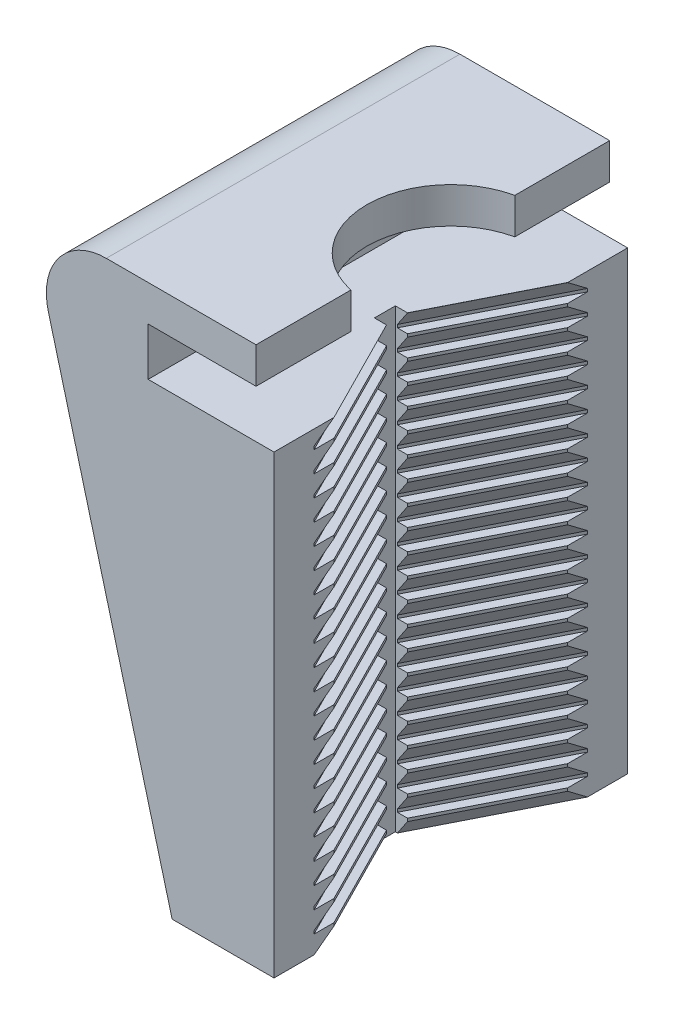
from build123d import *

# Parameters (mm, degrees)
BOSS_EXTRUDE1_DEPTH     = 59
CUT_EXTRUDE2_REACH      = 116.122
SKETCH3_R               = 14
CUT_EXTRUDE3_DEPTH      = 115.121756946
CUT_EXTRUDE3_DEPTH_BACK = 80
CUT_EXTRUDE5_DEPTH      = 80
CUT_EXTRUDE6_DEPTH      = 99.782303331
SKETCH9_W               = 3.123815153
SKETCH9_H               = 3.5
CUT_EXTRUDE7_DEPTH      = 80


with BuildPart() as part:
    # Sketch1 → Boss-Extrude1 (new body)
    with BuildSketch(Plane.XY):
        with BuildLine():
            Line((0, 0), (0, 76))
            Line((0, 76), (-21, 76))
            Line((-21, 76), (-21, 84))
            Line((-21, 84), (-3, 84))
            Line((-3, 84), (-3, 90))
            Line((-3, 90), (-27.983883536, 90))
            ThreePointArc((-27.983883536, 90), (-35.913772093, 86.092361404), (-37.646232932, 77.423373494))
            Line((-37.646232932, 77.423373494), (-17, 0))
            Line((-17, 0), (0, 0))
        make_face()
    extrude(amount=BOSS_EXTRUDE1_DEPTH)

    # Sketch3 → Cut-Extrude2 (cut, up to next)
    with BuildSketch(Plane(origin=(0, 90, 0), x_dir=(1, 0, 0), z_dir=(0, 1, 0)), mode=Mode.PRIVATE) as cut_extrude2_sk1:
        with Locations((0, -29.5)):
            Circle(SKETCH3_R)
    cut_extrude2_tool1 = extrude(cut_extrude2_sk1.sketch, amount=-CUT_EXTRUDE2_REACH, mode=Mode.PRIVATE) & part.part
    add(cut_extrude2_tool1.solids().sort_by_distance((0, 90, 29.5))[0], mode=Mode.SUBTRACT)

    # Sketch4 → Cut-Extrude3 (cut, two sides: drawn at the far end of the back side and taken through both)
    with BuildSketch(Plane(origin=(0, 0, 0), x_dir=(-1, 0, 0), z_dir=(0, -1, 0)).offset(-CUT_EXTRUDE3_DEPTH_BACK)):
        Polygon((9.393945477, -30.437233817), (0, -49), (0, -10), (9.393945477, -28.562766183), (11, -27.75), (11, -31.25), align=None)
    extrude(amount=CUT_EXTRUDE3_DEPTH + CUT_EXTRUDE3_DEPTH_BACK, mode=Mode.SUBTRACT)

    # Sketch7 → Cut-Extrude5 (cut)
    with BuildSketch(Plane(origin=(10.347410524, 0, 20.446846604), x_dir=(-0.8922525128420106, 0, 0.45153676852180913), z_dir=(-0.4515367685218092, 0, -0.8922525128420107))):
        Polygon((22.125301658, 2.5), (23.625301658, 0), (21.086592601, -2.199739596), (20.043900458, 77.689978498), (22.125301658, 76.5), (22.125301658, 76), (23.625301658, 73.5), (23.625301658, 73), (22.125301658, 73), (22.125301658, 72.5), (23.625301658, 70), (23.625301658, 69.5), (22.125301658, 69.5), (22.125301658, 69), (23.625301658, 66.5), (23.625301658, 66), (22.125301658, 66), (22.125301658, 65.5), (23.625301658, 63), (23.625301658, 62.5), (22.125301658, 62.5), (22.125301658, 62), (23.625301658, 59.5), (23.625301658, 59), (22.125301658, 59), (22.125301658, 58.5), (23.625301658, 56), (23.625301658, 55.5), (22.125301658, 55.5), (22.125301658, 55), (23.625301658, 52.5), (23.625301658, 52), (22.125301658, 52), (22.125301658, 51.5), (23.625301658, 49), (23.625301658, 48.5), (22.125301658, 48.5), (22.125301658, 48), (23.625301658, 45.5), (23.625301658, 45), (22.125301658, 45), (22.125301658, 44.5), (23.625301658, 42), (23.625301658, 41.5), (22.125301658, 41.5), (22.125301658, 41), (23.625301658, 38.5), (23.625301658, 38), (22.125301658, 38), (22.125301658, 37.5), (23.625301658, 35), (23.625301658, 34.5), (22.125301658, 34.5), (22.125301658, 34), (23.625301658, 31.5), (23.625301658, 31), (22.125301658, 31), (22.125301658, 30.5), (23.625301658, 28), (23.625301658, 27.5), (22.125301658, 27.5), (22.125301658, 27), (23.625301658, 24.5), (23.625301658, 24), (22.125301658, 24), (22.125301658, 23.5), (23.625301658, 21), (23.625301658, 20.5), (22.125301658, 20.5), (22.125301658, 20), (23.625301658, 17.5), (23.625301658, 17), (22.125301658, 17), (22.125301658, 16.5), (23.625301658, 14), (23.625301658, 13.5), (22.125301658, 13.5), (22.125301658, 13), (23.625301658, 10.5), (23.625301658, 10), (22.125301658, 10), (22.125301658, 9.5), (23.625301658, 7), (23.625301658, 6.5), (22.125301658, 6.5), (22.125301658, 6), (23.625301658, 3.5), (23.625301658, 3), (22.125301658, 3), align=None)
    extrude(amount=-CUT_EXTRUDE5_DEPTH, mode=Mode.SUBTRACT)

    # Sketch8 → Cut-Extrude6 (cut, through all)
    with BuildSketch(Plane(origin=(-13.42279364, 0, 26.52391165), x_dir=(0.8922525128420106, 0, 0.45153676852180913), z_dir=(-0.4515367685218092, 0, 0.8922525128420107))):
        Polygon((6.596768885, 77.671993362), (4.515367685, 76.482014864), (4.515367685, 75.982014864), (3.015367685, 73.482014864), (3.015367685, 72.982014864), (4.515367685, 72.982014864), (4.515367685, 72.482014864), (3.015367685, 69.982014864), (3.015367685, 69.482014864), (4.515367685, 69.482014864), (4.515367685, 68.982014864), (3.015367685, 66.482014864), (3.015367685, 65.982014864), (4.515367685, 65.982014864), (4.515367685, 65.482014864), (3.015367685, 62.982014864), (3.015367685, 62.482014864), (4.515367685, 62.482014864), (4.515367685, 61.982014864), (3.015367685, 59.482014864), (3.015367685, 58.982014864), (4.515367685, 58.982014864), (4.515367685, 58.482014864), (3.015367685, 55.982014864), (3.015367685, 55.482014864), (4.515367685, 55.482014864), (4.515367685, 54.982014864), (3.015367685, 52.482014864), (3.015367685, 51.982014864), (4.515367685, 51.982014864), (4.515367685, 51.482014864), (3.015367685, 48.982014864), (3.015367685, 48.482014864), (4.515367685, 48.482014864), (4.515367685, 47.982014864), (3.015367685, 45.482014864), (3.015367685, 44.982014864), (4.515367685, 44.982014864), (4.515367685, 44.482014864), (3.015367685, 41.982014864), (3.015367685, 41.482014864), (4.515367685, 41.482014864), (4.515367685, 40.982014864), (3.015367685, 38.482014864), (3.015367685, 37.982014864), (4.515367685, 37.982014864), (4.515367685, 37.482014864), (3.015367685, 34.982014864), (3.015367685, 34.482014864), (4.515367685, 34.482014864), (4.515367685, 33.982014864), (3.015367685, 31.482014864), (3.015367685, 30.982014864), (4.515367685, 30.982014864), (4.515367685, 30.482014864), (3.015367685, 27.982014864), (3.015367685, 27.482014864), (4.515367685, 27.482014864), (4.515367685, 26.982014864), (3.015367685, 24.482014864), (3.015367685, 23.982014864), (4.515367685, 23.982014864), (4.515367685, 23.482014864), (3.015367685, 20.982014864), (3.015367685, 20.482014864), (4.515367685, 20.482014864), (4.515367685, 19.982014864), (3.015367685, 17.482014864), (3.015367685, 16.982014864), (4.515367685, 16.982014864), (4.515367685, 16.482014864), (3.015367685, 13.982014864), (3.015367685, 13.482014864), (4.515367685, 13.482014864), (4.515367685, 12.982014864), (3.015367685, 10.482014864), (3.015367685, 9.982014864), (4.515367685, 9.982014864), (4.515367685, 9.482014864), (3.015367685, 6.982014864), (3.015367685, 6.482014864), (4.515367685, 6.482014864), (4.515367685, 5.982014864), (3.015367685, 3.482014864), (3.015367685, 2.982014864), (4.515367685, 2.982014864), (4.515367685, 2.482014864), (3.015367685, -0.017985136), (5.554076741, -2.217724732), align=None)
    extrude(amount=-CUT_EXTRUDE6_DEPTH, mode=Mode.SUBTRACT)

    # Sketch9 → Cut-Extrude7 (cut)
    with BuildSketch(Plane(origin=(0, 0, 0), x_dir=(-1, 0, 0), z_dir=(0, -1, 0))):
        with Locations((9.438092424, -29.5)):
            Rectangle(SKETCH9_W, SKETCH9_H)
    extrude(amount=-CUT_EXTRUDE7_DEPTH, mode=Mode.SUBTRACT)


solid = part.part
